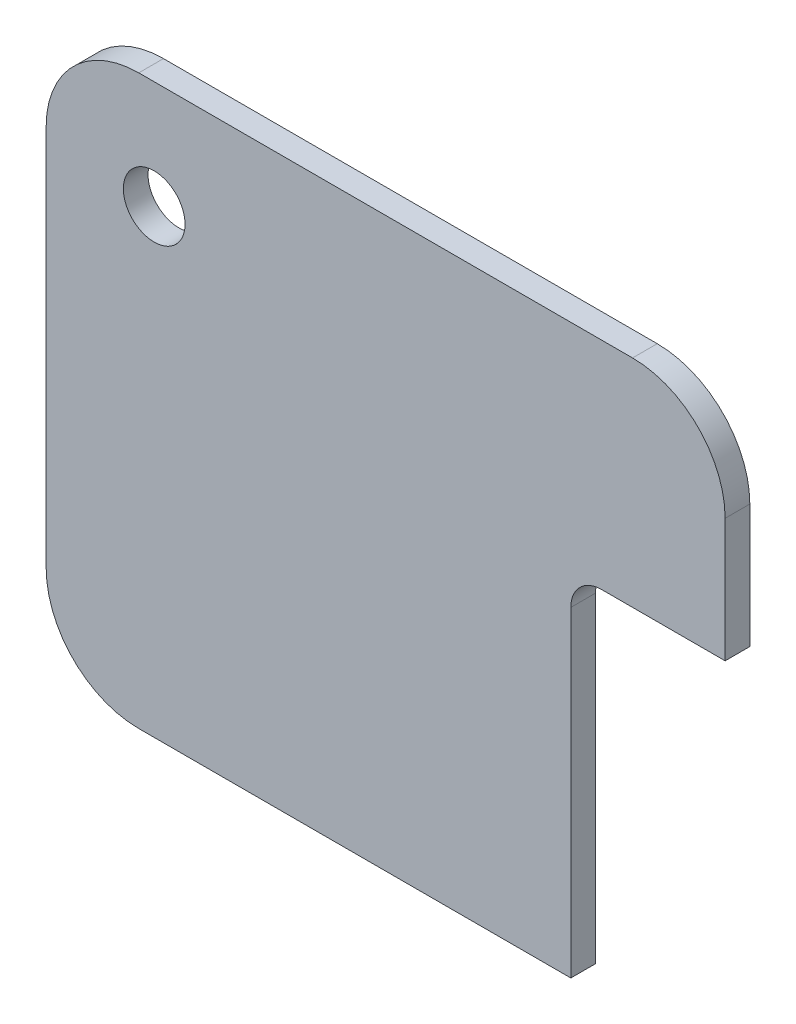
SolidWorks part; units mm, degrees
material "普通碳钢"
ref_plane "前视基准面" through (0, 0, 0) normal (0, 0, 1) x (1, 0, 0)
ref_plane "上视基准面" through (0, 0, 0) normal (0, 1, 0) x (1, 0, 0)
ref_plane "右视基准面" through (0, 0, 0) normal (1, 0, 0) x (0, 0, -1)
sketch "草图1" plane through (0, 0, 0) normal (0, 0, 1) x (1, 0, 0)
  line L0 (0, 30) -> (0, 154)
  line L1 (30, 184) -> (190, 184)
  line L2 (220, 154) -> (220, 114)
  line L3 (220, 114) -> (180, 114)
  line L4 (170, 104) -> (170, 0)
  line L5 (170, 0) -> (30, 0)
  arc A0 (190, 184) -> (220, 154) centre (190, 154) cw
  arc A1 (0, 30) -> (30, 0) centre (30, 30) ccw
  arc A2 (0, 154) -> (30, 184) centre (30, 154) cw
  arc A3 (180, 114) -> (170, 104) centre (180, 104) ccw
  circle A4 centre (35, 149) radius 10
  point P9 (220, 184)
  point P12 (0, 0)
  point P15 (0, 184)
  dimension "D5" = 30
  dimension "D6" = 10
  dimension "D9" = 20
  dimension "D1" = 220
  dimension "D2" = 70
  dimension "D3" = 184
  dimension "D4" = 170
  dimension "D7" = 35
  dimension "D8" = 35
extrude "凸台-拉伸1" add sketch "草图1" along normal blind 8
